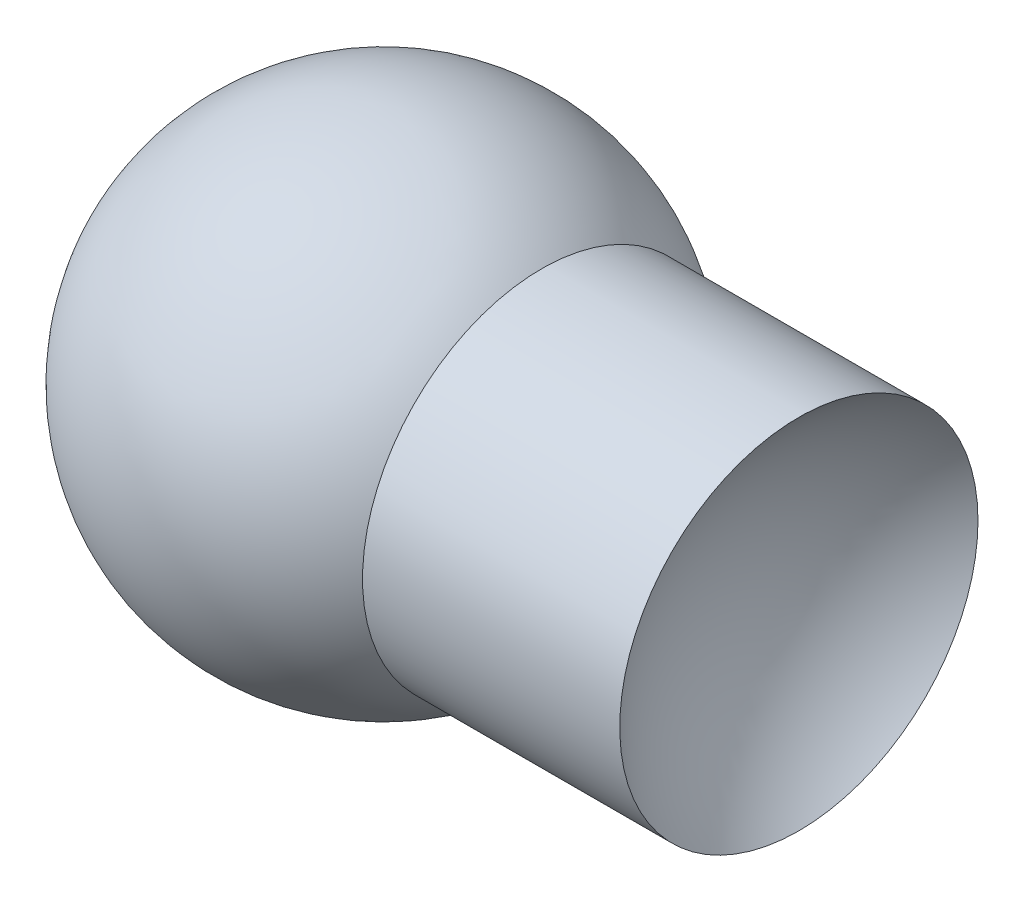
SolidWorks part; units mm, degrees
ref_plane "Front Plane" through (0, 0, 0) normal (0, 0, 1) x (1, 0, 0)
ref_plane "Top Plane" through (0, 0, 0) normal (0, 1, 0) x (1, 0, 0)
ref_plane "Right Plane" through (0, 0, 0) normal (1, 0, 0) x (0, 0, -1)
sketch "Sketch1" plane through (0, 0, 0) normal (0, 0, 1) x (1, 0, 0)
  line L0 (0, 23.7905) -> (0, -49976.2095) construction
  line L2 (0, 10) -> (0, -10)
  arc A0 (0, -10) -> (0, 10) centre (0, 0) ccw
  dimension "D1" = 20
revolve "Revolve3" add sketch "Sketch1" angle 360 about L0
sketch "Sketch2" plane through (0, 0, 0) normal (0, 0, 1) x (1, 0, 0)
  line L1 (11, 0) -> (-11, 0) construction
  line L2 (6.6144, 7.5) -> (17.3856, 7.5)
  line L3 (0, -11) -> (0, 11) construction
  line L4 (10, 0) -> (14, 0)
  line L5 (27.638, 0) -> (-49972.362, 0) construction
  line L7 (12, 15.5148) -> (12, -13.3598) construction
  circle A0 centre (0, 0) radius 10 construction
  arc A1 (10, 0) -> (6.6144, 7.5) centre (0, 0) ccw
  arc A2 (14, 0) -> (17.3856, 7.5) centre (24, 0) cw
  dimension "D1" = 7.5
  dimension "D2" = 14
revolve "Revolve4" add sketch "Sketch2" angle 360 about L5
